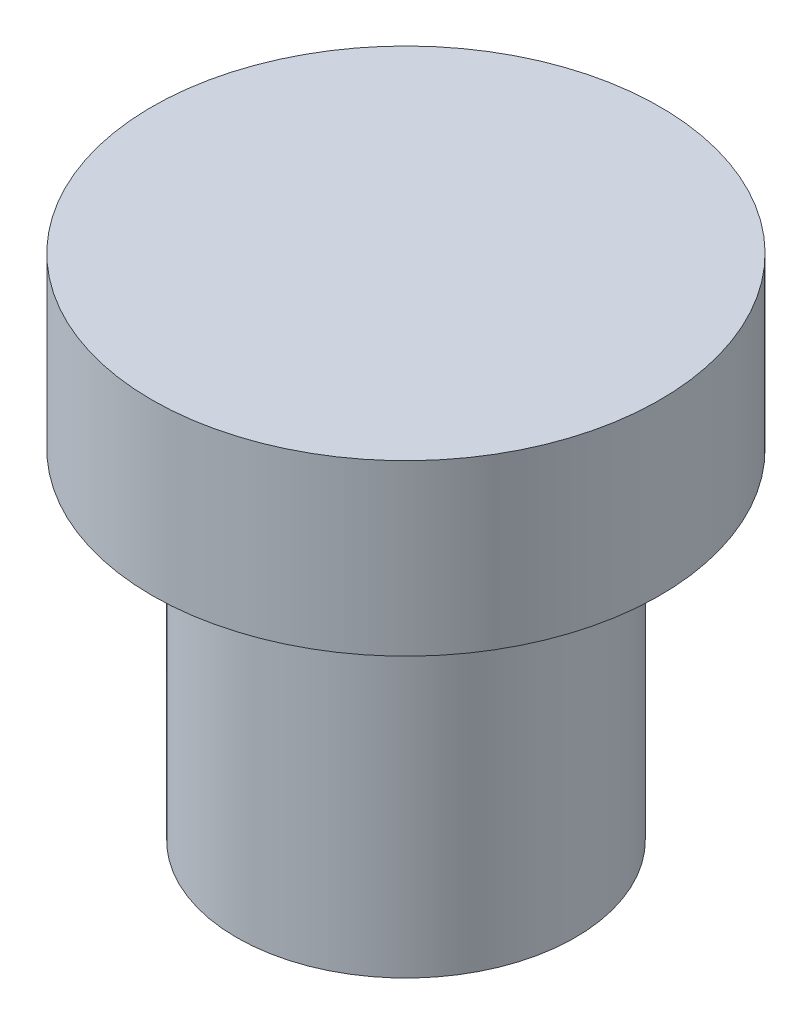
SolidWorks part; units mm, degrees
ref_plane "Front Plane" through (0, 0, 0) normal (0, 0, 1) x (1, 0, 0)
ref_plane "Top Plane" through (0, 0, 0) normal (0, 1, 0) x (1, 0, 0)
ref_plane "Right Plane" through (0, 0, 0) normal (1, 0, 0) x (0, 0, -1)
sketch "Sketch1" plane through (0, 0, 0) normal (0, 1, 0) x (1, 0, 0)
  circle A0 centre (0, 0) radius 5
  dimension "D1" = 10
extrude "Boss-Extrude1" add sketch "Sketch1" along normal blind 10
sketch "Sketch2" plane through (0, 10, 0) normal (0, 1, 0) x (1, 0, 0)
  circle A0 centre (0, 0) radius 7.5
  dimension "D1" = 15
extrude "Boss-Extrude2" add sketch "Sketch2" along normal blind 5
